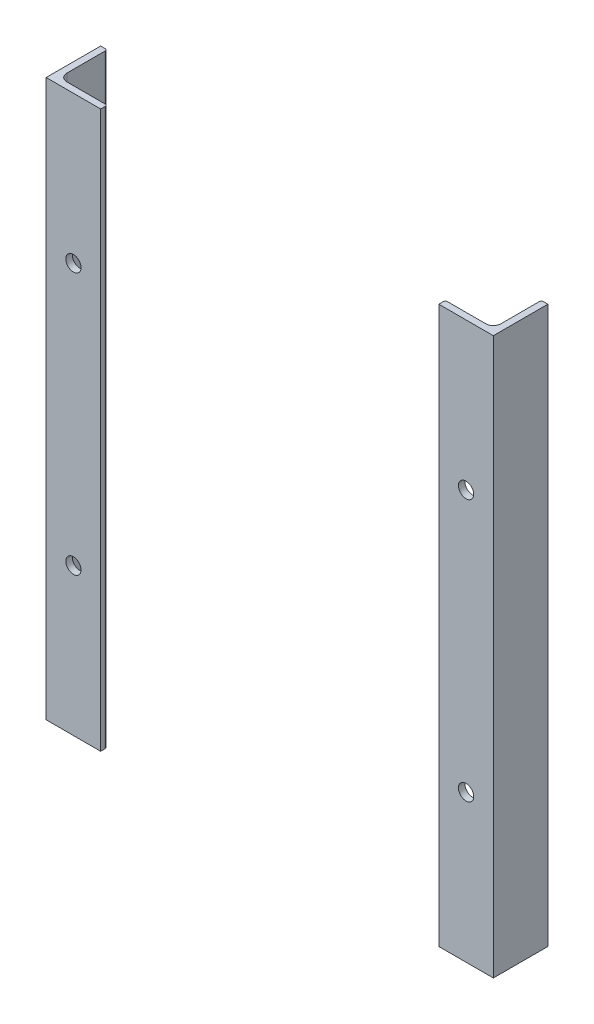
from build123d import *

# Parameters (mm, degrees)
EQUAL_ANGLE_2_5X3_1_DEPTH     = 255
EQUAL_ANGLE_2_5X3_1_2_DEPTH   = 255
M6_CLEARANCE_HOLE1_AT_2_COUNT = 2
M6_CLEARANCE_HOLE1_AT_2_PITCH = 120
M6_CLEARANCE_HOLE1_AT_3_COUNT = 2
M6_CLEARANCE_HOLE1_AT_3_PITCH = 216.333076528
M6_CLEARANCE_HOLE1_AT_4_COUNT = 2
M6_CLEARANCE_HOLE1_AT_4_PITCH = 180


with BuildPart() as part:
    # Sketch1 → Equal Angle 2.5X3(1) (new body)
    with BuildSketch(Plane(origin=(-102.5, -127.5, 0), x_dir=(0, 0, -1), z_dir=(0, 1, 0))):
        with BuildLine():
            Line((25, 0), (0, 0))
            Line((0, 0), (0, -25))
            Line((0, -25), (2, -25))
            ThreePointArc((2, -25), (2.707106781, -24.707106781), (3, -24))
            Line((3, -24), (3, -6.5))
            ThreePointArc((3, -6.5), (4.025126266, -4.025126266), (6.5, -3))
            Line((6.5, -3), (24, -3))
            ThreePointArc((24, -3), (24.707106781, -2.707106781), (25, -2))
            Line((25, -2), (25, 0))
        make_face()
    extrude(amount=EQUAL_ANGLE_2_5X3_1_DEPTH)

    # Sketch6 → M6 Clearance Hole1 (revolve, cut)
    with BuildSketch(Plane(origin=(-90, 60, 0), x_dir=(0, -1, 0), z_dir=(1, 0, 0))):
        Polygon((0, 0), (0, 22.103012167), (3.5, 20), (3.5, 0), align=None)
    m6_clearance_hole1 = revolve(axis=Axis((-90, 60, 6.35), (0, 0, -1)), mode=Mode.SUBTRACT)

    # M6 Clearance Hole1 at 2: M6 Clearance Hole1 ×2
    with Locations(*[(0, -i * M6_CLEARANCE_HOLE1_AT_2_PITCH, 0) for i in range(1, M6_CLEARANCE_HOLE1_AT_2_COUNT)]):
        add(m6_clearance_hole1, mode=Mode.SUBTRACT)


with BuildPart() as body_2:
    # Sketch1 on segment 2 (carried to segment 2) → Equal Angle 2.5X3_1 2 (new body)
    with BuildSketch(Plane(origin=(102.5, -127.5, 0), x_dir=(-1, 0, 0), z_dir=(0, 1, 0))):
        with BuildLine():
            Line((25, 0), (0, 0))
            Line((0, 0), (0, -25))
            Line((0, -25), (2, -25))
            ThreePointArc((2, -25), (2.707106781, -24.707106781), (3, -24))
            Line((3, -24), (3, -6.5))
            ThreePointArc((3, -6.5), (4.025126266, -4.025126266), (6.5, -3))
            Line((6.5, -3), (24, -3))
            ThreePointArc((24, -3), (24.707106781, -2.707106781), (25, -2))
            Line((25, -2), (25, 0))
        make_face()
    extrude(amount=EQUAL_ANGLE_2_5X3_1_2_DEPTH)

    # M6 Clearance Hole1 at 3: M6 Clearance Hole1 ×2
    with Locations(*[Vector(0.8320502943378437, -0.5547001962252293, 0) * (i * M6_CLEARANCE_HOLE1_AT_3_PITCH) for i in range(1, M6_CLEARANCE_HOLE1_AT_3_COUNT)]):
        add(m6_clearance_hole1, mode=Mode.SUBTRACT)

    # M6 Clearance Hole1 at 4: M6 Clearance Hole1 ×2
    with Locations(*[(i * M6_CLEARANCE_HOLE1_AT_4_PITCH, 0, 0) for i in range(1, M6_CLEARANCE_HOLE1_AT_4_COUNT)]):
        add(m6_clearance_hole1, mode=Mode.SUBTRACT)


solid = Compound([part.part, body_2.part])
